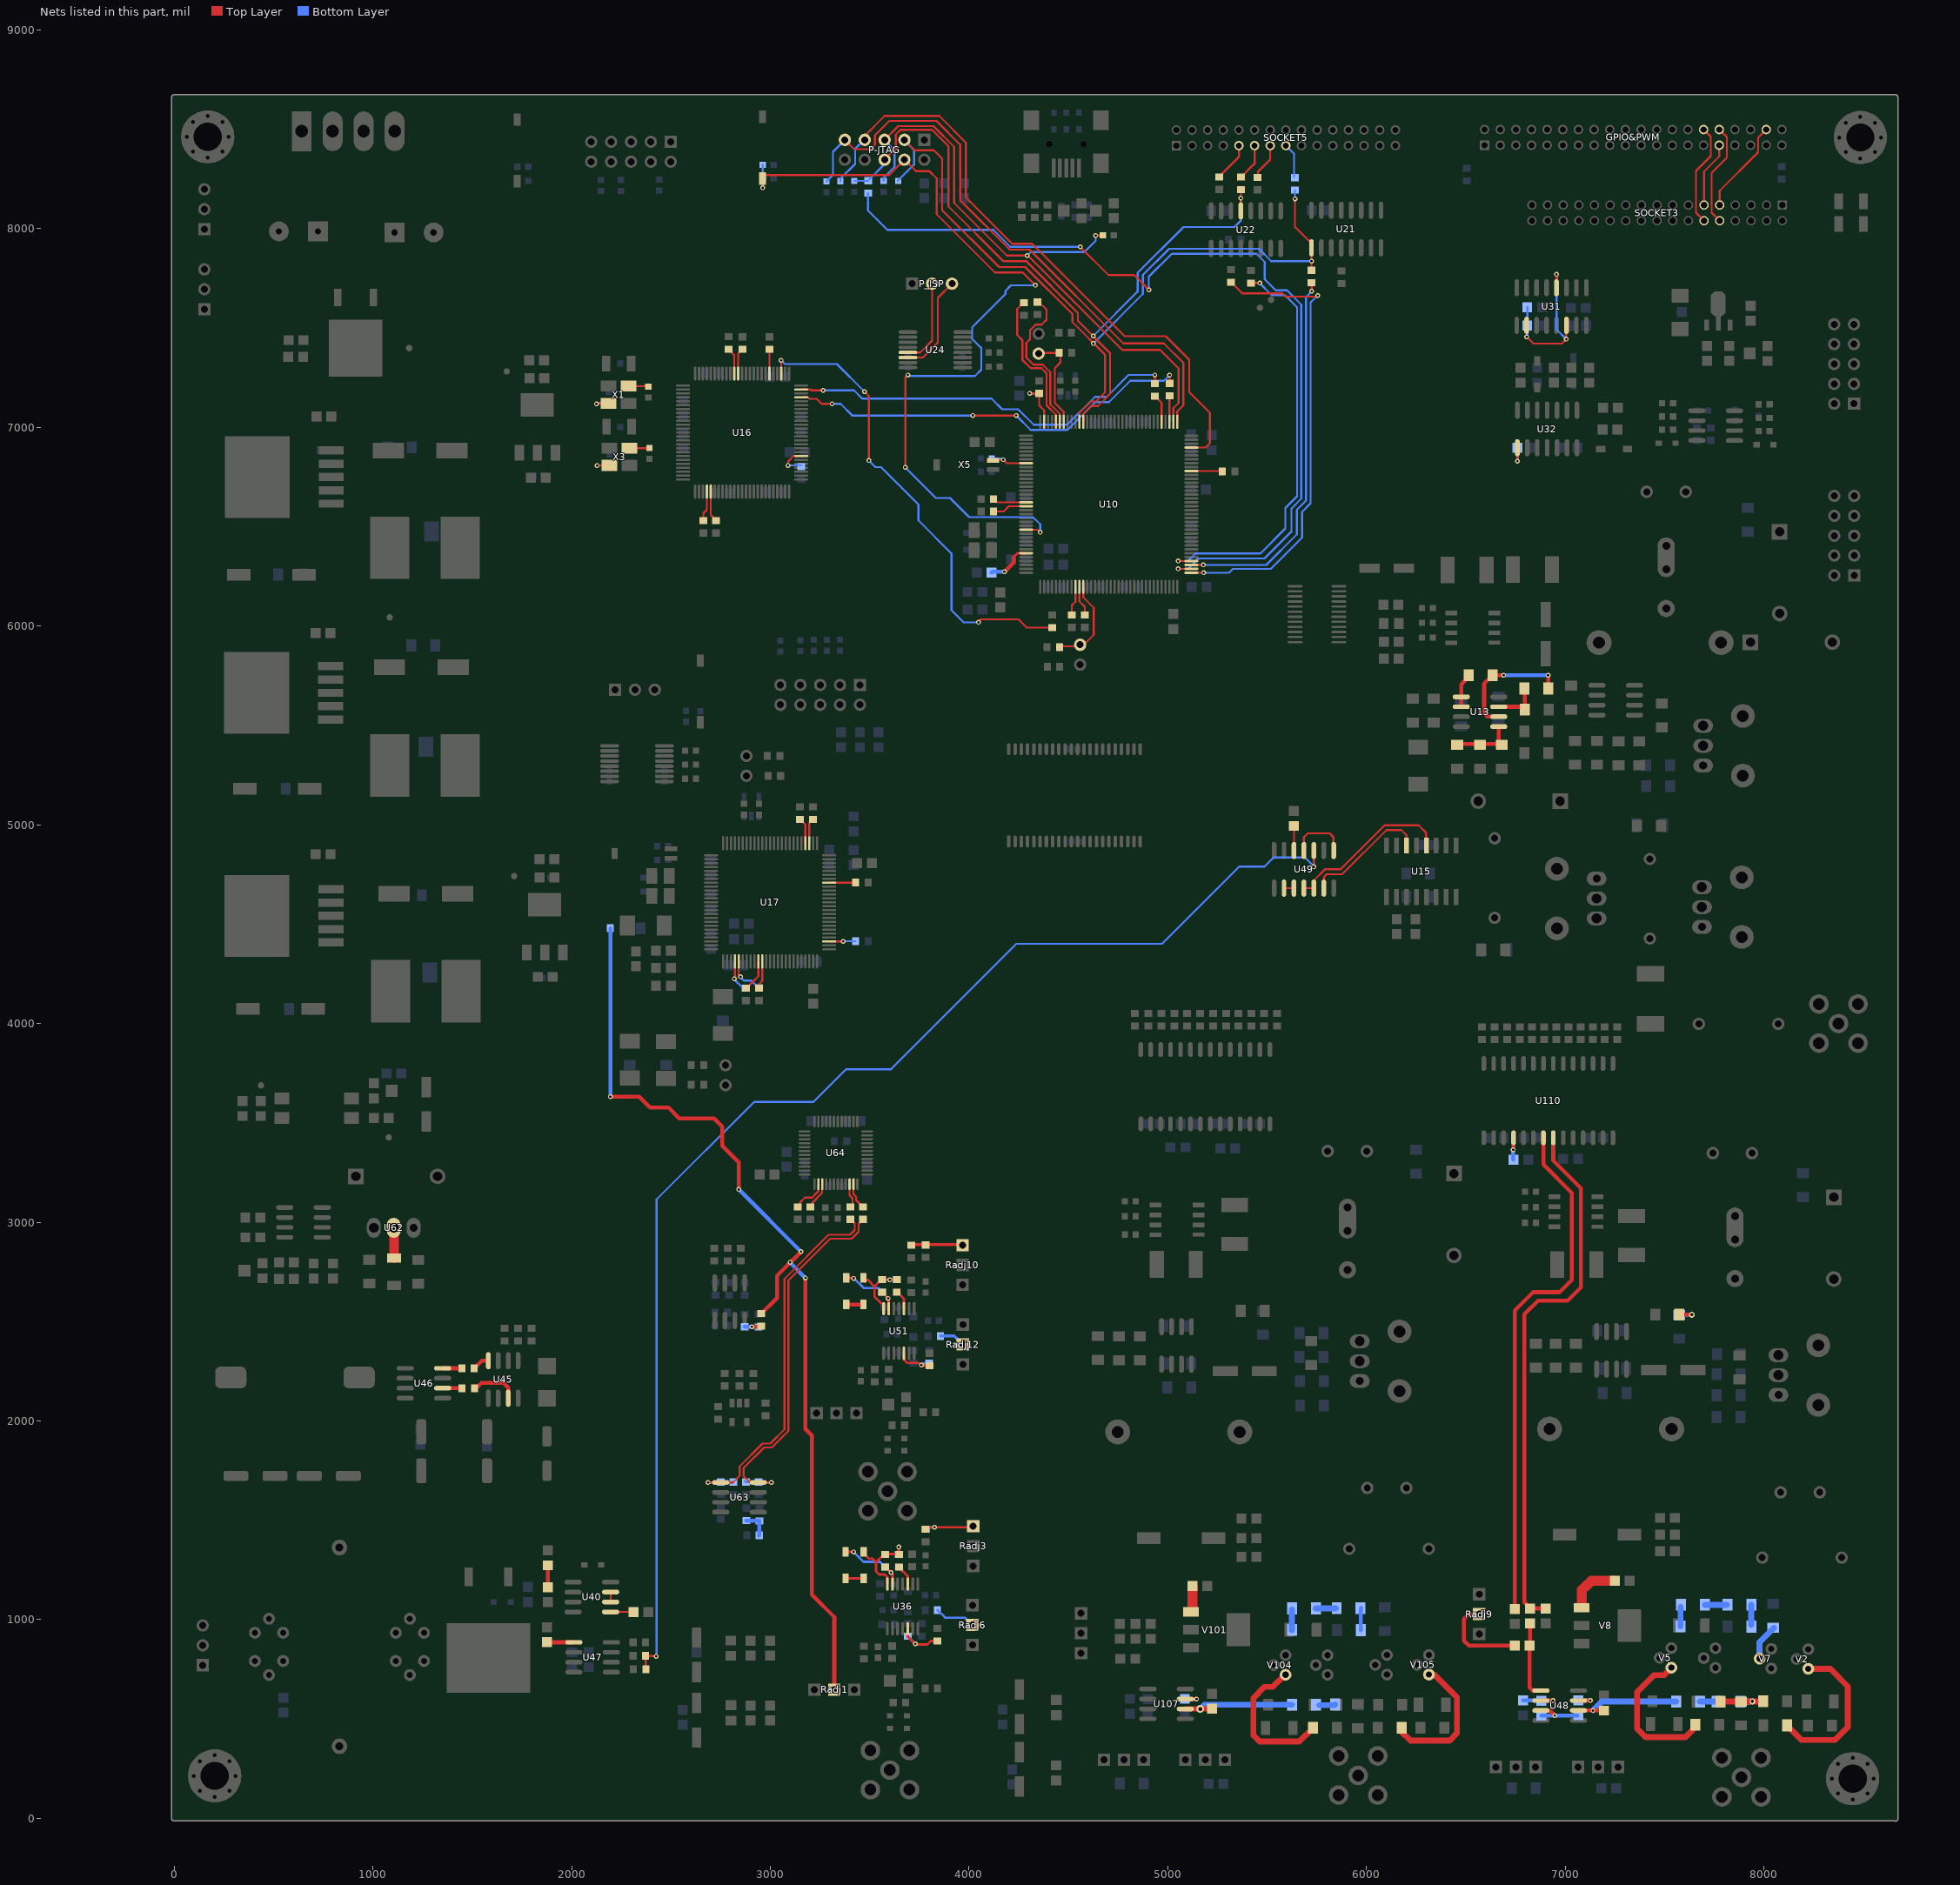
[diagram p0: the nets of this part, all layers, seen from the top]
# Altium PCB MISC82309.PcbDoc (part 11 of 14)
Units mil, origin at the board's own origin, x right, y up, seen from the top; angles counter-clockwise.
Board outline 8687.03 x 8687.86 mil, 4 copper layers (Top Layer, GND, POWER, Bottom Layer); 747 components, 583 nets, 2530 pads, 1834 vias.

## Via types
v1: diameter 24, hole 12, Top Layer to Bottom Layer, 1799 vias
v2: diameter 30, hole 15, Top Layer to Bottom Layer, 26 vias
v3: diameter 40, hole 20, Top Layer to Bottom Layer, 9 vias

## Nets (pads, with @x,y where several pads share a name; then routed paths per layer and width w, separated by ;. In a path a pad name is that pad's centre, name@x,y a point inside that pad or via, vN(x,y) a via of type N, cw(c..) or ccw(c..) an arc to the next point about the centre after c; other vN are vias at no path point) (continued)
NetR44_1: R44.1 V101.1 | length 126.2
  Top Layer w50: R44.1@5124.5,1170 5124.5,1097 5124.5,1044.5 V101.1@5125,1044
NetR47_2: R47.2 U107.3 | length 101.5
  Top Layer w20: U107.3@5088.49,601 v1(5145,601)
  Bottom Layer w20: R47.2@5100,601 v1(5145,601)
NetR48_2: R48.2 R163.2 U107.2 | length 600.6
  Top Layer w20: R48.2@5213,551 R48.2@5215,549
  Top Layer w25: U107.2@5088.49,551 R48.2@5213,551
  Bottom Layer w30: v3(5163,551) 5165,551 5166,552 5165,552 5165,553 5184,572 R163.2@5625,572
NetR58_1: R58.1 X1.1 | length 126.3
  Top Layer w10: v1(2125,7119) 2127,7121 X1.1@2187,7121
  Bottom Layer w10: v1(2125,7119) 2128.5,7122.5 R58.1@2187,7122.5
NetR59_2: R59.2 X1.3 | length 99.9
  Top Layer w10: X1.3@2287,7207.61 2383.89,7207.61 R59.2@2386,7205.5
NetR70_1: R70.1 U13.1 U13.2 | length 152.8
  Top Layer w20: U13.2@6476.51,5594 U13.1@6476.51,5644 6476.51,5706.51 R70.1@6505,5735
NetR70_2: R70.2 R80.1 U13.6 | length 649.9
  Top Layer w20: R70.2@6628,5734 R70.2@6646,5752 ; R70.2@6634,5753 6592,5711 6592,5561 6609,5544 U13.6@6661,5544 ; R70.2@6642,5753 v1(6690,5753) ; R80.1@6914,5686 v1(6914,5753)
  Bottom Layer w20: v1(6690,5753) v1(6914,5753)
NetR71_2: R71.2 R73.2 R79.2 U13.5 | length 284
  Top Layer w20: R79.2@6470,5404 6472,5406 6664.98,5406 6665.49,5406.51 U13.5@6665.49,5494
NetR78_1: R78.1 R80.2 U13.7 | length 227.9
  Top Layer w20: U13.7@6665.49,5594 6790,5594 R78.1@6796,5588 ; R78.1@6796,5580 R78.1@6796,5588 ; R80.2@6796,5670 R78.1@6796,5588 ; R78.1@6799.5,5584.5 R78.1@6796,5588
NetR101_2: R101.2 SOCKET5.9 | length 196.8
  Top Layer w10: R101.2@5263,8260.5 5263,8266 5357.96,8360.96 SOCKET5.9@5357.96,8418
NetR102_2: R102.2 SOCKET5.11 | length 186.5
  Top Layer w10: R102.2@5369,8259.5 5436.7,8327.2 SOCKET5.11@5436.7,8418
NetR103_2: R103.2 SOCKET5.13 | length 188.4
  Top Layer w10: R103.2@5448,8257.5 5454,8263.5 5454,8286 5515.44,8347.44 SOCKET5.13@5515.44,8418
NetR104_2: R104.2 SOCKET5.15 | length 171.4
  Bottom Layer w10: SOCKET5.15@5594.18,8418 5635,8377.18 R104.2@5635,8263.5
NetR108_1: R108.1 X3.1 | length 124.6
  Top Layer w10: v1(2129,6808) 2130,6809 X3.1@2191,6809
  Bottom Layer w10: v1(2129,6808) 2129.5,6808.5 R108.1@2191,6808.5
NetR109_2: R109.2 X3.3 | length 101.4
  Top Layer w10: X3.3@2291,6895.61 2391.11,6895.61 R109.2@2392,6896.5
NetR152_2: R152.2 V105.1 | length 708.4
  Top Layer w20: V105.1@6316,728 V105.1@6328,728
  Top Layer w30: R152.2@6177,456 6177,436 6221,392 6418,392 6455,429 6455,610 6342,723 V105.1@6318,723
NetR153_1: R153.1 R154.2 | length 113.2
  Bottom Layer w20: R153.1@5971,947 5971,1056 R154.2@5974,1059
NetR154_1: R154.1 R161.2 | length 102.4
  Bottom Layer w20: R154.1@5846,1057 R154.1@5847,1056
  Bottom Layer w30: R161.2@5745,1057 R154.1@5846,1057
NetR155_2: R155.2 R156.1 U31.4 U31.10 U31.14 | length 912.9
  Top Layer w10: U31.10@6806,7513.51 v1(6806,7456) 6840,7422 6983,7422 v1(7005,7444) 7005,7512.51 U31.14@7006,7513.51 ; U31.4@6956,7702.49 v1(6956,7770)
  Bottom Layer w10: v1(6806,7456) 6809.5,7459.5 6809.5,7513 R155.2@6809.5,7604 ; v1(6956,7770) 6956,7493 v1(7005,7444)
NetR161_1: R161.1 R162.2 | length 104.8
  Bottom Layer w20: R161.1@5623,1052 R161.1@5625,1050
  Bottom Layer w30: R162.2@5625,948 R161.1@5625,1050
NetR163_1: R163.1 R164.2 | length 82.2
  Bottom Layer w30: R163.1@5761,570 5839,570 R164.2@5842,573
NetR189_2: R189.2 R191.2 R193.2 U36.14 V11.1 | length 398.3
  Top Layer w12: V11.1@3482,1322 3497,1307 3515,1307 3532,1290 ; R191.2@3562,1320 3532,1290 ; R191.2@3578,1328 3580,1330 3646,1330 v1(3646,1366) ; U36.14@3589.23,1179.2 3589.23,1213.77 3575,1228 3548,1228 3532,1244 3532,1290
  Bottom Layer w12: R189.2@3646,1328.5 v1(3646,1366)
NetR190_2: R190.2 R191.1 U36.13 V10.1 | length 328.2
  Top Layer w12: V10.1@3379,1341.93 3414.93,1341.93 v1@3415,1342 ; R191.1@3590,1254 3607,1237 v1(3608,1237) ; U36.13@3614.82,1179.2 v1@3614.82,1229.18
  Bottom Layer w12: v1(3419,1341) 3469,1291 3551.5,1291 R190.2@3577,1265.5 ; R190.2@3589,1257 3589,1256 v1(3608,1237)
NetR193_1: R193.1 U36.10 | length 103.4
  Top Layer w12: R193.1@3649,1265 3649,1261 3691.59,1218.41 U36.10@3691.59,1179.2
NetR195_1: R195.1 R196.1 Radj3.1 | length 282.7
  Top Layer w12: R196.1@3788,1465 v1(3826,1465) 4016,1465 Radj3.1@4021,1470 ; Radj3.1@4013.5,1455.5 Radj3.1@4015,1457
  Bottom Layer w12: R195.1@3782,1455.5 3790.5,1464 v1@3824,1464
NetR198_2: R198.2 R199.1 U36.5 | length 259.7
  Top Layer w12: U36.5@3691.59,954.8 3691.59,913.41 3730,875 3790.36,875 3808.36,893 R199.1@3832,893
  Bottom Layer w12: R198.2@3691,916.5 3728.5,879 v1(3730,879)
NetR200_2: R200.2 Radj6.2 | length 180.1
  Bottom Layer w12: R200.2@3841.5,1048 3879.5,1010 3979,1010 Radj6.2@3998,991
NetR203_1: R203.1 V104.1 | length 734.8
  Top Layer w20: R203.1@5731,450 R203.1@5731,456
  Top Layer w30: V104.1@5584,718 5528,662 5487,662 5431,606 5431,418 5462,387 5662,387 R203.1@5731,456
NetR212_1: R212.1 U32.8 | length 135
  Top Layer w10: v1(6759,6830) U32.8@6759,6897.51
  Bottom Layer w10: v1(6759,6830) R212.1@6759,6897.5
NetR213_1: R213.1 U46.2 | length 97
  Top Layer w20: U46.2@1351.49,2165 R213.1@1448.5,2165
NetR213_2: R213.2 U45.7 | length 244.1
  Top Layer w20: R213.2@1511.5,2165 1520,2165 1547,2192 1657,2192 1681,2168 U45.7@1681,2114.51
NetR214_1: R214.1 U46.4 | length 96
  Top Layer w20: U46.4@1351.49,2265 R214.1@1447.5,2265
NetR214_2: R214.2 U45.4 | length 86.4
  Top Layer w20: R214.2@1510.5,2265 1548.98,2303.49 U45.4@1581,2303.49
NetR215_2: R215.2 U47.5 | length 134.7
  Top Layer w20: R215.2@1877,886.5 1877.5,886 U47.5@2011.51,886
NetR216_1: R216.1 R217.1 | length 110.4
  Top Layer w20: R217.1@1880,1273.5 1881,1272.5 R216.1@1881,1163.5
NetR220_1: R220.1 U40.5 | length 115
  Top Layer w10: U40.5@2196.49,1039 R220.1@2311.5,1039
NetR227_2: R227.2 R236.1 | length 108
  Top Layer w20: R227.2@7574,2535 v2(7637,2535)
  Bottom Layer w20: R236.1@7592,2535 v2(7637,2535)
NetR274_1: R274.1 R275.2 U10.143 | length 249.3
  Top Layer w10: v1(4305.01,7171.01) R274.1@4353,7171.01 4353,7111 4378.2,7085.8 U10.143@4378.2,7028.35
  Bottom Layer w10: v1(4305.01,7171.01) 4352.5,7171.01 R275.2@4353,7171.5
NetR287_2: R287.2 R288.1 U49.10 | length 6535.2
  Top Layer w10: R287.2@2373.5,751 2373.5,816.5 2374,817 v1@2426,817 ; v1(5735,4789) U49.10@5735,4870.49
  Bottom Layer w10: v1@2428,818 2428,3115 2919,3606 3217,3606 3381,3770 3607,3770 4238,4401 4971,4401 5360,4790 5487,4790 5533,4836 5690,4836 v1@5735,4791
  other v1: 2426,816
NetR290_1: R290.1 R320.2 U48.7 | length 261.8
  Top Layer w20: U48.7@6877.51,543 6921,543 v1(6947,517)
  Bottom Layer w20: R320.2@6879,517.5 R290.1@7060.5,517.5
NetR290_2: R290.2 U48.3 | length 114
  Top Layer w20: U48.3@7066.49,593 v1(7126,593)
  Bottom Layer w20: R290.2@7066,593.5 v1@7120.5,593.5
NetR291_1: R291.1 V8.1 | length 265
  Top Layer w50: V8.1@7083,1069 7083,1149 7100,1166 ; 7101,1165 7131,1195 R291.1@7249.5,1195
NetR292_2: R292.2 R305.2 U48.2 | length 566.2
  Top Layer w20: U48.2@7066.49,543 v1(7139,543) R292.2@7195,543
  Bottom Layer w20: v1(7139,543) v1@7141,545
  Bottom Layer w30: v1@7141,545 7184,588 R305.2@7558,588
NetR297_1: R297.1 V7.2 | length 172.8
  Bottom Layer w30: V7.2@7977,816 7977,887 R297.1@8049,959
NetR298_2: R298.2 R299.1 R302.1 R306.1 | length 267.4
  Top Layer w30: R298.2@7789,589 R299.1@7996,589
  Bottom Layer w30: R306.1@7882,588 7883,589 v2(7942,589)
NetR303_1: R303.1 V5.1 | length 743.7
  Top Layer w30: V5.1@7528,751 7498,721 7447,721 7361,635 7361,452 7404,409 7606,409 7654,457 R303.1@7654,472
NetR304_2: R304.2 V2.1 | length 799.4
  Top Layer w30: R304.2@8117,468 8117,466 8188,395 8358,395 8422,459 8422,664 8334,752 V2.1@8227,752
NetR305_1: R305.1 R306.2 | length 84.4
  Bottom Layer w30: R305.1@7678,588 7761,588 R306.2@7762,587
NetR307_1: R307.1 R308.2 | length 101
  Bottom Layer w30: R307.1@7936,974 R308.2@7936,1075
NetR308_1: R308.1 R309.2 | length 110
  Bottom Layer w30: R309.2@7703,1075 R308.1@7813,1075
NetR309_1: R309.1 R310.2 | length 98
  Bottom Layer w30: R310.2@7580,966 R309.1@7580,1064
NetR314_1: R314.1 U110.21 | length 2627.7
  Top Layer w20: R314.1@6737,1061 R314.1@6738,1060 ; R314.1@6746,1054.5 6746,2556 6838,2648 6972,2648 7032,2708 7032,3149 6890,3291 U110.21@6890,3424.99
NetR315_2: R315.2 R320.1 U48.6 | length 218.2
  Top Layer w20: U48.6@6877.51,593 v1(6938,593)
  Bottom Layer w20: R315.2@6788,593.5 R320.1@6885.5,593.5 ; R320.1@6879,592.5 6938.5,592.5 v1@6939,593
NetR316_2: R316.2 R317.1 U110.22 | length 2708.3
  Top Layer w20: R316.2@6891,1057 6826,1057 6795,1088 6795,2537 6863,2605 7012,2605 7079,2672 7079,3171 6940,3310 U110.22@6940,3424.99
NetR317_2: R317.2 R321.2 U48.5 | length 378.3
  Top Layer w20: R321.2@6821.5,869 6821.5,657.5 6836,643 U48.5@6867,643 ; R317.2@6823,980.5 6823,868 R321.2@6825,866
NetR318_1: R318.1 U110.18 | length 106.9
  Top Layer w20: v1(6738,3365) 6740,3367 U110.18@6740,3424.99
  Bottom Layer w20: v1@6737,3360 6737,3317.5 R318.1@6739.5,3315
NetR321_1: R321.1 Radj9.2 | length 462.5
  Top Layer w20: Radj9.2@6564,1026 6512,1026 6490,1004 6490,894 6515,869 R321.1@6746.5,869 ; Radj9.2@6588,1027.5 Radj9.2@6588,1030
NetR325_2: R325.2 R327.2 R329.2 U51.14 V12.1 | length 351
  Top Layer w12: V12.1@3469,2709 3492,2709 3524,2677 ; R327.2@3549,2702 3524,2677 ; U51.14@3570.23,2565.2 3570.23,2579.77 3524,2626 3524,2677
  Top Layer w15: R327.2@3563,2711.5 v1@3602,2711.5 ; v1(3602,2711) v1@3602,2711.5 ; R329.2@3634,2713 3632.5,2711.5 v1@3602,2711.5 ; R329.2@3636,2711.5 R329.2@3644,2719.5
  Bottom Layer w15: v1(3602,2711) R325.2@3635,2711
NetR326_2: R326.2 R327.1 U51.13 V13.1 | length 350.1
  Top Layer w12: V13.1@3382.07,2720 3420,2720 v1@3421,2719 ; R327.1@3571,2640 3595.82,2615.18 U51.13@3595.82,2565.2
  Bottom Layer w12: v1@3420,2719 3469.75,2669.25 3543.75,2669.25 R326.2@3563.75,2649.25 ; R326.2@3552,2646 3564,2646 v1(3593,2617)
  other v1: 3419,2718
NetR329_1: R329.1 U51.10 | length 92.1
  Top Layer w12: R329.1@3643,2645 3672.59,2615.41 U51.10@3672.59,2565.2
NetR331_1: R331.1 R332.1 Radj10.1 | length 237.7
  Top Layer w10: Radj10.1@3954,2885.5 3955.5,2885.5 Radj10.1@3956,2886
  Top Layer w15: R331.1@3721,2888 3722,2887 Radj10.1@3954,2887 ; R332.1@3782,2885.5 R332.1@3783.5,2887
NetR334_2: R334.2 R339.1 U51.5 | length 216.7
  Top Layer w12: U51.5@3672.59,2340.8 3672.59,2309.41 3690,2292 3714,2292 3747,2292 3761,2278 R339.1@3801,2278
  Bottom Layer w12: v1(3760,2281) 3769.5,2290.5 R334.2@3800,2290.5
NetR336_2: R336.2 Radj12.2 | length 114.2
  Bottom Layer w15: R336.2@3856.5,2428 3924,2428 Radj12.2@3957,2395
NetR345_1: R345.1 U16.29 | length 152.6
  Top Layer w10: R345.1@2663,6531.5 2663,6568 2680.83,6585.83 U16.29@2680.83,6676.76
NetR346_1: R346.1 U16.30 | length 156.2
  Top Layer w10: U16.30@2700.52,6676.76 2700.52,6559.48 2727,6533 R346.1@2727,6531.5
NetR347_1: R347.1 U16.81 | length 121.3
  Top Layer w10: U16.81@2995.8,7271.24 2995.8,7392.3 R347.1@2996,7392.5
NetR348_1: R348.1 U10.47 | length 152.6
  Top Layer w10: U10.47@4555.36,6197.65 4555.36,6124.64 4583,6097 R348.1@4583,6056.5
NetR349_1: R349.1 U10.46 | length 148.9
  Top Layer w10: R349.1@4517,6056.5 4517,6104 4535.68,6122.68 U10.46@4535.68,6197.65
NetR386_1: R386.1 U49.12 | length 110.5
  Top Layer w10: U49.12@5635,4870.49 R386.1@5635,4981
NetR391_1: R391.1 U10.19 | length 175
  Top Layer w10: R391.1@4123.5,6577 4174,6577 4200.16,6603.16 U10.19@4287.65,6603.16
NetR392_1: R392.1 U10.18 | length 168.8
  Top Layer w10: R392.1@4123.5,6639.17 R392.1@4129,6639.17 ; R392.1@4129,6634 4140.16,6622.84 U10.18@4287.65,6622.84
NetR405_1: R405.1 U10.73 | length 2348.8
  Top Layer w10: U10.73@5118.35,6268.51 v1(5180.51,6268.51) ; R405.1@5320,7729 5375,7674 5576,7674 5592,7658 5749,7658 v1(5755,7664)
  Bottom Layer w10: v1(5180.51,6268.51) 5308.51,6268.51 5328,6288 5518,6288 5676,6446 5676,6575 5719,6618 5719,7628 v1(5755,7664)
NetR406_1: R406.1 U10.74 | length 4582.5
  Top Layer w10: v1(4560,7909) 4560,7908 4702,7766 4832,7766 4904.5,7693.5 v1(4904.5,7691.5) ; v1(5052.2,6288.2) U10.74@5118.35,6288.2
  Bottom Layer w10: R406.1@3492,8178.5 3492,8091 3589,7994 4122,7994 4207,7909 v1@4559,7909 ; v1@4560,7908 v1(4560,7909) ; v1(4904.5,7691.5) 4904.5,7758.5 5020,7874 5446,7874 5488,7832 5488,7746 5544,7690 5600,7690 5672,7618 5672,6641 5622,6591 5622,6476 5486,6340 5154,6340 5102.2,6288.2 v1(5052.2,6288.2)
NetR407_1: R407.1 U10.75 | length 1884.6
  Top Layer w10: U10.75@5118.35,6307.88 v1(5178.88,6307.88) ; v1@5724,7692 R407.1@5724,7727.5
  Bottom Layer w10: v1(5178.88,6307.88) 5495.88,6307.88 5650,6462 5650,6586 5696,6632 5696,7657 5705,7666 v1(5724,7685)
NetR408_1: R408.1 U10.76 | length 2091.4
  Top Layer w10: v1(5051.57,6327.57) U10.76@5118.35,6327.57 ; R408.1@5418,7726.5 v1@5458.5,7726.5
  Bottom Layer w10: v1(5051.57,6327.57) 5101.57,6327.57 5140,6366 5467,6366 5592,6491 5592,6594 5651,6653 5651,7604 5589,7666 5523,7666 v1(5463,7726)
NetR409_1: R409.1 U16.89 | length 130.7
  Top Layer w10: U16.89@2838.32,7271.24 2838.32,7369.82 R409.1@2861,7392.5
NetR410_1: R410.1 U16.90 | length 134.5
  Top Layer w10: R410.1@2789,7393.5 2818.63,7363.87 U16.90@2818.63,7271.24
NetR411_1: R411.1 R412.2 R478.2 | length 101.8
  Top Layer w20: v1(2907,2474) R478.2@2939,2474
  Bottom Layer w20: R412.2@2871,2474.02 2905,2474.02 v1(2907,2474) 2938.02,2474.02 R411.1@2940,2476
NetR415_2: R415.2 U64.3 | length 134.4
  Top Layer w10: R415.2@3212,3077.5 3212,3099.37 3261.1,3148.47 U64.3@3261.1,3191.52
NetR416_1: R416.1 U64.2 | length 173.4
  Top Layer w10: R416.1@3149,3077.5 3149,3099 3174,3124 3210,3124 3241.42,3155.42 U64.2@3241.42,3191.52
NetR418_1: R418.1 U64.10 | length 116
  Top Layer w10: 3398.9,3136 U64.10@3398.9,3191.52 ; 3399,3136 3414,3121 3414,3110 3414,3105 3414,3086 R418.1@3411,3083
NetR419_2: R419.2 U64.11 | length 133.5
  Top Layer w10: 3418.58,3142 U64.11@3418.58,3191.52 ; 3419,3142 3419,3141 3431.25,3128.75 3431.25,3112.25 R419.2@3466,3077.5
NetR455_1: R455.1 U16.57 | length 156.9
  Top Layer w10: v1@3090,6816 3090,6829 3116.89,6855.89 U16.57@3155.24,6855.89
  Bottom Layer w10: v1(3088.5,6808.5) R455.1@3156,6808.5
NetR478_1: R478.1 R556.2 Radj1.2 | length 4907
  Top Layer w20: v1(2195,3632) 2340,3632 2395,3577 2488,3577 2542,3523 2716,3523 2758,3481 2758,3384 2841,3301 v1(2841,3165) ; R478.1@2951.5,2536.5 3034,2619 3034,2731 v1@3156,2853 ; v1(3177,2720) 3177,1960 3209.5,1927.5 3209.5,1125.5 3322,1013 Radj1.2@3322,648
  Bottom Layer w20: v1@2195.5,3635 R556.2@2195.5,4479 ; v1@2841,3166 v1@3153.5,2853.5 ; v1(3100,2799) 3100,2797 v1(3177,2720) ; v1@3155,2852 v1(3155,2853)
NetR508_1: R508.1 U10.99 | length 166.3
  Top Layer w10: U10.99@5118.35,6780.32 5284.18,6780.32 R508.1@5284.5,6780
NetR509_2: R509.2 U10.111 | length 130.5
  Top Layer w10: U10.111@5008.12,7028.35 5008.12,7157.62 R509.2@5009,7158.5
NetR511_2: R511.2 U10.113 | length 141.7
  Top Layer w10: R511.2@4936,7156.5 4968.75,7123.76 U10.113@4968.75,7028.35
NetR513_1: R513.1 U17.78 | length 127.8
  Top Layer w10: U17.78@3195.85,4907.24 3195.85,5009.35 R513.1@3214,5027.5
NetR514_1: R514.1 U17.79 | length 131.1
  Top Layer w10: R514.1@3150,5027.5 3176.17,5001.34 U17.79@3176.17,4907.24
NetR515_1: R515.1 U17.35 | length 162.4
  Top Layer w10: R515.1@2877,4178.5 2880.44,4178.5 2913,4211.06 2913.06,4211.06 2939.94,4237.94 U17.35@2939.94,4312.76
NetR516_1: R516.1 U17.36 | length 141.1
  Top Layer w10: R516.1@2943,4178.5 2944,4179.5 2944,4199 2959.63,4214.63 U17.36@2959.63,4312.76
NetR518_1: R518.1 U17.68 | length 133.5
  Top Layer w10: U17.68@3296.24,4708.43 3428.93,4708.43 R518.1@3429.5,4709
NetR519_1: R519.1 U17.53 | length 133.7
  Top Layer w10: U17.53@3296.24,4413.15 3366.85,4413.15 v1(3367,4413)
  Bottom Layer w10: v1(3367,4413) 3368,4414 R519.1@3429.5,4414
NetR521_1: R521.1 R522.2 R578.2 | length 142.4
  Bottom Layer w20: R522.2@2879,1498.5 2943.5,1498.5 R578.2@2945,1500 ; R521.1@2942,1423 2945,1426 R578.2@2945,1497.5
NetR558_2: R558.2 U16.78 | length 2400
  Top Layer w10: U16.78@3054.85,7271.24 v1(3054.85,7337.85) ; v1(3474,7180) 3496,7158 v1(3496,6833) ; v1@4049,6023 4060,6034 4249,6034 4290.5,5992.5 R558.2@4418,5992.5
  Bottom Layer w10: v1(3054.85,7337.85) 3073.7,7319 3335,7319 v1(3474,7180) ; v1(3496,6833) 3529,6800 3557,6800 3745,6612 3745,6532 3912,6365 3912,6080 3973,6019 v1(4047,6019)
NetR564_2: R564.2 U17.30 | length 196.1
  Top Layer w10: U17.30@2841.52,4312.76 2840.5,4311.74 2840.5,4244.5 v1(2850,4235) v1@2851,4235
  Bottom Layer w10: v1@2851,4232 2867,4216 2904,4216 R564.2@2934,4186 ; R564.2@2935.25,4187.25 R564.2@2943,4179.5
NetR565_2: R565.2 U17.29 | length 157.7
  Top Layer w10: v1@2821.83,4225.83 U17.29@2821.83,4312.76
  Bottom Layer w10: v1(2819,4225) 2819,4222.06 2862.06,4179 R565.2@2869,4179
NetR567_1: R567.1 U10.139 | length 775.6
  Top Layer w10: R567.1@4352,7631 4390,7593 4390,7542 4365,7517 4336,7517 4333,7514 4332.19,7514 4307,7488.81 4307,7444 4288,7425 4288,7352 4324,7316 4371.04,7316 4409,7278.04 4409,7116.04 4456.94,7068.1 U10.139@4456.94,7028.35
NetR569_1: R569.1 U10.140 | length 728.6
  Top Layer w10: 4268,7399 4268,7393 ; R569.1@4272,7626 4242,7596 4242,7465 4268,7439 4268,7393 ; U10.140@4437.25,7028.35 4437.25,7063.75 4390,7111 4390,7273 4365,7298 4311,7298 4268,7341 4268,7393
NetU15_12: U15.12 U49.4 U49.5 | length 832.8
  Top Layer w10: U49.4@5685,4681.51 U49.5@5735,4681.51 ; U49.5@5737,4682 5736.51,4681.51 U49.5@5735,4681.51 ; 6299,4961 6262.5,4997.5 6090.5,4997.5 5869,4776 5791,4776 5735,4720 U49.5@5735,4681.51 ; U15.12@6300,4913 6300,4961
NetU15_14: U15.14 U49.6 | length 609.8
  Top Layer w10: U49.6@5785,4681.51 5785,4736 5800,4751 5877,4751 6100,4974 6175,4974 6201,4948 U15.14@6201,4918
NetU40_6: U40.6 U40.7 | length 50
  Top Layer w10: U40.6@2196.49,1089 U40.7@2196.49,1139
NetU49_2: U49.2 U49.3 | length 50.5
  Top Layer w10: U49.2@5585,4681.51 U49.3@5635,4681.51 U49.3@5635.51,4681.51
NetU49_8: U49.8 U49.11 | length 269.3
  Top Layer w10: U49.11@5685,4870.49 5685,4938 5704,4957 5815,4957 5834,4938 U49.8@5834,4901
NetU62_2: U62.2 V1.2 | length 150.1
  Top Layer w50: V1.2@1107,2819.9 U62.2@1107,2970
NetV10_2: V10.2 V11.2 | length 89.4
  Top Layer w12: V10.2@3379,1208.07 3466.93,1208.07 V11.2@3468,1207
NetV12_2: V12.2 V13.2 | length 74.9
  Top Layer w20: V13.2@3391.07,2586 V12.2@3466,2586
OE_A: R509.1 U16.72 | length 2075.6
  Top Layer w10: U16.72@3155.24,7151.17 3190.41,7151.17 3197.57,7144 3233,7144 3259,7118 v1(3311,7118) ; v1(4019,7060) v1(4237,7060) ; R509.1@5009,7221.5 v1(5009,7263)
  Bottom Layer w10: v1@3313,7118 3354,7118 3412,7060 v1(4019,7060) ; v1(4237,7060) 4310,6987 4495,6987 4635,7127 4704,7127 4811,7234 4980,7234 v1(5009,7263)
OE_B: R511.1 U16.74 | length 2002.4
  Top Layer w10: U16.74@3155.24,7190.54 3202.46,7190.54 3206.78,7186.22 3261.78,7186.22 v1@3265,7183 ; v1(4935,7264) 4936,7263 R511.1@4936,7219.5
  Bottom Layer w10: v1(3266,7186) 3421,7186 3462,7145 4113.54,7145 4167,7091.54 4246.46,7091.54 4325,7013 4493,7013 4634,7154 4693,7154 4803,7264 v1(4935,7264)
OUT+: C501.1 R419.1 R523.1 U63.4 | length 1907.1
  Top Layer w10: v1(3005,1691) U63.4@2939.49,1691 2897,1691 2866,1722 2866,1763.72 2969,1866.72 3008,1866.72 3091,1949.72 3091,2707 3301,2917 3409,2917 3444.5,2952.5 3444.5,2991.5 3466,3013 R419.1@3466,3014.5
  Bottom Layer w10: C501.1@2872,1697 2876.5,1692.5 C501.1@2878,1692.5 R523.1@2942,1692.5 ; R523.1@2950,1694 2953,1691 v1(3005,1691)
OUT-: C502.1 R418.2 R524.1 U63.5 | length 1921.6
  Top Layer w10: v1(2687,1691) U63.5@2750.51,1691 2813,1691 2846,1724 2846,1752 ; 2846,1750 2846,1752 ; R418.2@3403,3014.5 3403.5,3014.5 3424.5,2993.5 3424.5,2960.78 3400.72,2937 3292.72,2937 3071,2715.28 3071,1958 2999.72,1886.72 2960.72,1886.72 2846,1772 2846,1752
  Bottom Layer w10: v1(2687,1691) R524.1@2750,1691 ; R524.1@2750.51,1692.5 2805.5,1692.5 C502.1@2808,1695
OUTPUT0: GPIO&PWM.31 SOCKET3.11 | length 332.8
  Top Layer w10: SOCKET3.11@7698.3,8119 7698.3,8287.3 7775.1,8364.1 GPIO&PWM.31@7775.1,8420
OUTPUT1: GPIO&PWM.30 SOCKET3.12 | length 520.6
  Top Layer w10: GPIO&PWM.30@7696.36,8498.74 7732,8463.1 7732,8365 7658,8291 7658,8080.56 SOCKET3.12@7698.3,8040.26
OUTPUT2: GPIO&PWM.38 SOCKET3.9 | length 476.8
  Top Layer w10: SOCKET3.9@7777.04,8119 7777.04,8191.04 7971,8385 7971,8458.42 GPIO&PWM.38@8011.32,8498.74
OUTPUT3: GPIO&PWM.32 SOCKET3.10 | length 522.2
  Top Layer w10: GPIO&PWM.32@7775.1,8498.74 7813,8460.84 7813,8357 7737,8281 7737,8080.3 SOCKET3.10@7777.04,8040.26
P_AGND: R269.1 U10.31 | length 235.9
  Top Layer w10: 4225,6345 4227.5,6347.5
  Top Layer w12: 4226,6349 4243.94,6366.94 U10.31@4287.65,6366.94
  Top Layer w20: v1(4178,6274) 4179,6273 4225,6319 4225,6345 4225,6347
  Bottom Layer w20: R269.1@4113.5,6268.51 4117.99,6273 4179,6273 v1(4178,6274)
P_BOOT0: P_BOOT0.2 R64.1 U10.138 | length 487.1
  Top Layer w10: P_BOOT0.2@4351,7375 4460.5,7375 4460.5,7327.5 4431.25,7298.25 4431.25,7159.78 4432,7159.03 4432,7123.06 4476.62,7078.44 U10.138@4476.62,7028.35
P_BOOT1: P_BOOT1.2 R65.1 U10.48 | length 464.2
  Top Layer w10: R65.1@4457,5898 P_BOOT1.2@4561.5,5898 ; P_BOOT1.2@4560,5888 4628,5956 4628,6092 4575.05,6144.95 U10.48@4575.05,6197.65
P_ISP_RX: P_ISP.2 U24.13 | length 432.6
  Top Layer w10: U24.13@3692.2,7377.2 3754.2,7377.2 3814,7437 P_ISP.2@3814,7723
P_ISP_TX: P_ISP.3 U24.14 | length 507.4
  Top Layer w10: U24.14@3692.2,7351.61 3767.61,7351.61 3843,7427 3843,7652 P_ISP.3@3914,7723
P_JNTRST: P-JTAG.3 R104.1 R407.2 R589.1 U10.134 U21.1 | length 4061.6
  Top Layer w10: P-JTAG.3@3675,8447 3727,8395 3823,8395 3865,8353 3865,8093 4151,7807 4283,7807 4520,7570 4520,7530 4685,7365 4685,7178 4638,7131 4614,7131 4555.36,7072.36 U10.134@4555.36,7028.35 ; v1(5640,8150) 5640,8009 U21.1@5720,7929 ; U21.1@5723,7903.51 v1(5723,7836) 5723,7800 R407.2@5726,7797
  Bottom Layer w10: R589.1@3643,8240.5 3643,8242 3723,8322 3723,8398 P-JTAG.3@3688,8433 ; v1(4625,7422) 4875,7672 4875,7733.96 4874.5,7734.46 4874.5,7748.54 4875,7749.04 4875,7767 5007,7899 5458,7899 5521,7836 v1(5723,7836) ; v1(5640,8150) R104.1@5640,8193.5
P_JTCK: P-JTAG.9 R591.2 U10.109 | length 3025.2
  Top Layer w10: P-JTAG.9@3375,8447 3422,8400 3504,8400 3527,8423 3527,8470 3599,8542 3836,8542 3955,8423 3955,8144 4205,7894 4305,7894 4776,7423 4980,7423 5078,7325 5078,7111 5047.49,7080.49 U10.109@5047.49,7028.35
  Bottom Layer w10: R591.2@3283,8238.5 3315,8270.5 3315,8387 P-JTAG.9@3370,8442
P_JTDI: P-JTAG.5 R149.1 R587.1 U10.110 | length 3136.3
  Top Layer w10: P-JTAG.5@3575,8447 3644,8516 3821,8516 3925,8412 3925,8130 4190,7865 4296,7865 4771,7390 4961,7390 5054,7297 5054,7123 5027.8,7096.8 U10.110@5027.8,7028.35 ; v1(4637,7966) R149.1@4673.5,7966
  Bottom Layer w10: R587.1@3570,8240.5 3570,8256 3625,8311 3625,8395 P-JTAG.5@3580,8440 ; v1(4293,7865) 4310,7882 4580,7882 4637,7939 v1(4637,7966)
P_JTDO: P-JTAG.6 R102.1 R406.2 R590.1 U10.133 U22.13 | length 3789.4
  Top Layer w10: P-JTAG.6@3575,8347 3632,8404 3632,8473 3657,8498 3813,8498 3896,8415 3896,8112 4171,7837 4287,7837 4547.76,7576.24 ; 4547.52,7575.99 4547.52,7536.44 4710,7373.96 4710,7169 4649,7108 4617,7108 4575.05,7066.05 U10.133@4575.05,7028.35 ; U22.13@5368,8089.49 v1(5368,8154) R102.1@5368,8198
  Bottom Layer w10: R590.1@3423,8240.5 3492.5,8240.5 R406.2@3493,8240 ; R406.2@3492,8241.5 3576,8325.5 P-JTAG.6@3576,8341 ; v1(4625,7460) 4848,7683 4848,7777 5079,8008 5335,8008 5368,8041 v1(5368,8154)
P_JTMS: P-JTAG.7 R588.1 U10.105 | length 3187.4
  Top Layer w10: P-JTAG.7@3475,8447 3475,8467 3575,8567 3850,8567 3984,8433 3984,8157 4217,7924 4318,7924 4783,7459 4990,7459 5108,7341 5108,7178 5212,7074 5212,6920 5190.43,6898.43 U10.105@5118.35,6898.43
  Bottom Layer w10: R588.1@3353,8239.5 3353,8252 3427,8326 3427,8402 P-JTAG.7@3472,8447
P_NRST: C39.2 P-JTAG.4 P_REST.1 R63.2 U10.25 | length 4352.2
  Top Layer w10: P_REST.1@2961.17,8253 2961.17,8205.83 v1(2961.5,8205.5) ; P_REST.1@2961.17,8270 3598,8270 P-JTAG.4@3675,8347 3732,8290 3799,8290 3837,8252 3837,8073 4131,7779 4270,7779 v1(4334,7715) ; v1(3679,6799) 3680,6800 3680,7252 v1(3692,7264) ; U10.25@4287.65,6485.05 4344.95,6485.05 v1(4358,6472) v1@4364.91,6472
  Bottom Layer w10: v1(2961.5,8205.5) R63.2@2961.5,8253 C39.2@2961.5,8321 ; v1(3679,6799) 3833,6645 3904,6645 4000.58,6548.42 4321.58,6548.42 4358,6512 v1(4358,6472) ; v1@3697,7259 4030,7259 4061.5,7290.5 4061.5,7399.5 4049,7412 ; 4050.5,7410.5 4049,7412 ; v1(4334,7715) 4211.06,7715 4183,7686.94 4183,7671 4016,7504 4016,7445 4049,7412
P_OSC32_IN: C98.2 U10.8 X5.1 | length 233.1
  Top Layer w10: X5.1@4121,6834.62 4174.62,6834.62 4189.55,6819.69 U10.8@4287.65,6819.69
  Bottom Layer w10: C98.2@4114.5,6844 4165.24,6844 v1(4171.95,6837.29)